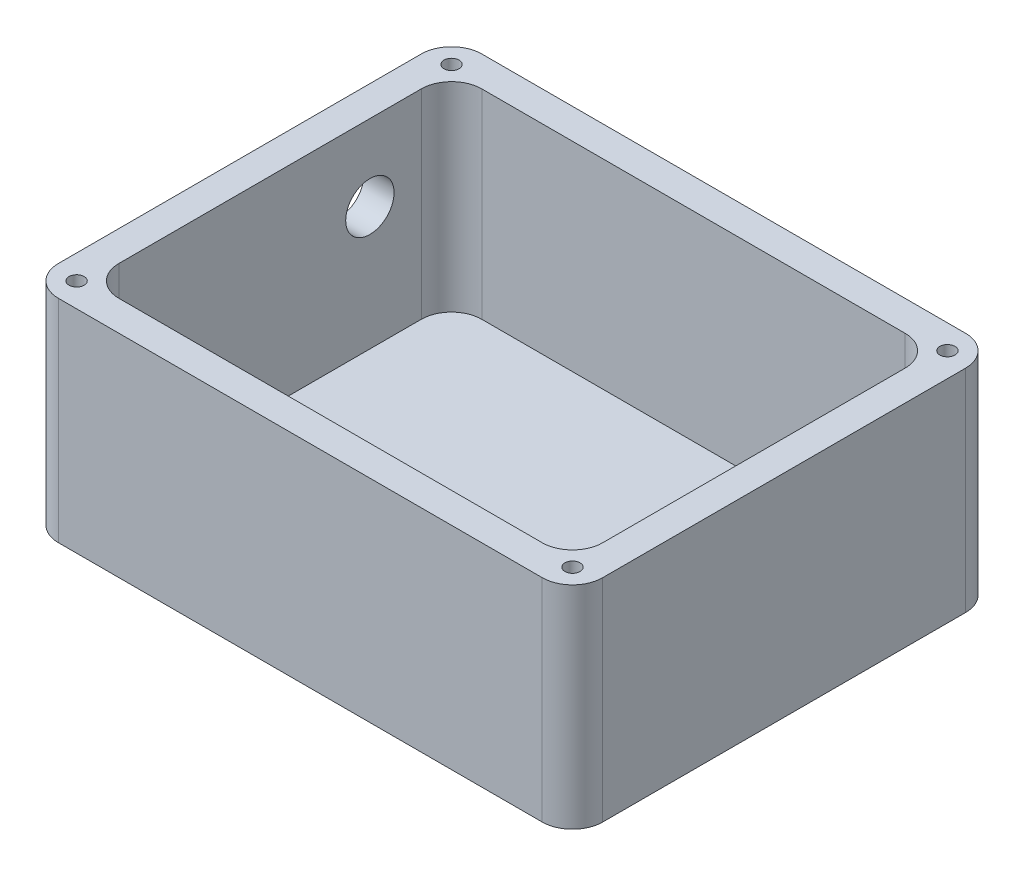
from build123d import *

# Parameters (mm, degrees)
SKETCH1_W             = 90
SKETCH1_H             = 70
BOSS_EXTRUDE1_DEPTH   = 35
SKETCH2_W             = 80
SKETCH2_H             = 60
CUT_EXTRUDE1_DEPTH    = 33
FILLET1_R             = 5
M3_TAPPED_HOLE1_D     = 2.5
M3_TAPPED_HOLE1_DEPTH = 8.5
M3_TAPPED_HOLE1_TIP   = 0.751075774
SKETCH7_R             = 4
CUT_EXTRUDE2_DEPTH    = 10


with BuildPart() as part:
    # Sketch1 → Boss-Extrude1 (new body)
    with BuildSketch(Plane(origin=(0, 0, 0), x_dir=(1, 0, 0), z_dir=(0, 1, 0))):
        Rectangle(SKETCH1_W, SKETCH1_H)
    extrude(amount=BOSS_EXTRUDE1_DEPTH)

    # Sketch2 → Cut-Extrude1 (cut)
    with BuildSketch(Plane(origin=(0, 35, 0), x_dir=(1, 0, 0), z_dir=(0, 1, 0))):
        Rectangle(SKETCH2_W, SKETCH2_H)
    extrude(amount=-CUT_EXTRUDE1_DEPTH, mode=Mode.SUBTRACT)

    # Fillet1
    fillet1_edges = [part.edges().sort_by_distance(p)[0] for p in [
        (40, 18.5, -30),
        (40, 18.5, 30),
        (-40, 18.5, 30),
        (-40, 18.5, -30),
        (45, 17.5, 35),
        (-45, 17.5, 35),
        (-45, 17.5, -35),
        (45, 17.5, -35),
    ]]
    fillet(fillet1_edges, radius=FILLET1_R)

    # M3 Tapped Hole1
    with Locations(Plane(origin=(0, 35, 0), x_dir=(1, 0, 0), z_dir=(0, 1, 0))):
        with Locations((-41, 31), (41, 31), (41, -31), (-41, -31)):
            Hole(M3_TAPPED_HOLE1_D / 2, depth=M3_TAPPED_HOLE1_DEPTH)
            with Locations((0, 0, -(M3_TAPPED_HOLE1_DEPTH + M3_TAPPED_HOLE1_TIP / 2))):  # 118° drill point
                Cone(0, M3_TAPPED_HOLE1_D / 2, M3_TAPPED_HOLE1_TIP, mode=Mode.SUBTRACT)

    # Sketch7 → Cut-Extrude2 (cut)
    with BuildSketch(Plane.ZY.offset(45)):
        with Locations((-16.5, 22.4)):
            Circle(SKETCH7_R)
    extrude(amount=-CUT_EXTRUDE2_DEPTH, mode=Mode.SUBTRACT)


solid = part.part
